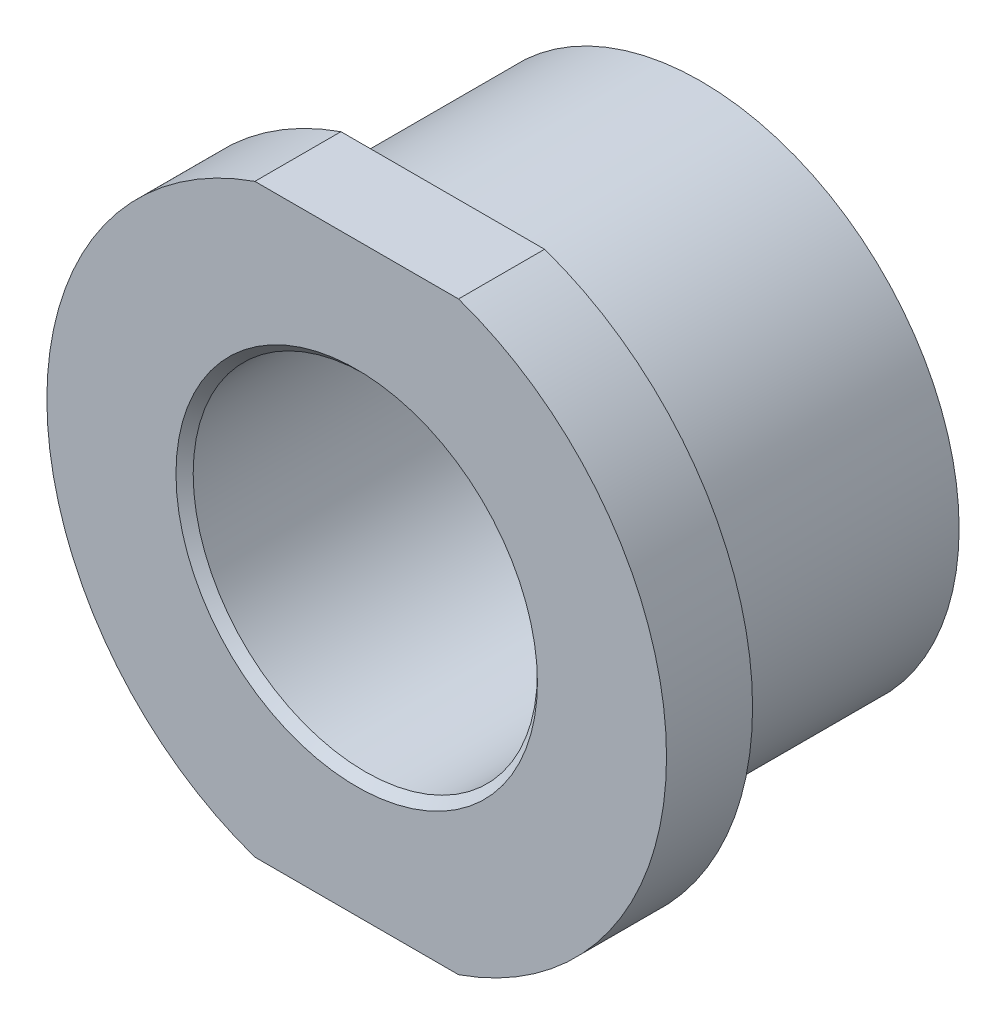
SolidWorks part; units mm, degrees
ref_plane "Front Plane" through (0, 0, 0) normal (0, 0, 1) x (1, 0, 0)
ref_plane "Top Plane" through (0, 0, 0) normal (0, 1, 0) x (1, 0, 0)
ref_plane "Right Plane" through (0, 0, 0) normal (1, 0, 0) x (0, 0, -1)
sketch "Sketch1" plane through (0, 0, 0) normal (0, 0, 1) x (1, 0, 0)
  circle A0 centre (0, 0) radius 15
  circle A1 centre (0, 0) radius 10
  dimension "D1" = 30
  dimension "D2" = 20
extrude "Boss-Extrude1" add sketch "Sketch1" along normal blind 15
sketch "Sketch2" plane through (0, 0, 15) normal (0, 0, 1) x (1, 0, 0)
  line L0 (-5.9161, 17) -> (5.9161, 17)
  line L1 (-5.9161, -17) -> (5.9161, -17)
  circle A0 centre (0, 0) radius 10 construction
  circle A1 centre (0, 0) radius 10
  arc A2 (-5.9161, 17) -> (-5.9161, -17) centre (0, 0) ccw
  arc A3 (5.9161, -17) -> (5.9161, 17) centre (0, 0) ccw
  dimension "D1" = 36
  dimension "D2" = 34
  dimension "D3" = 17
extrude "Boss-Extrude2" add sketch "Sketch2" along normal blind 5
chamfer "Chamfer1" distance 0.5 angle 45 2 edges at (10, 0, 0) (10, 0, 20)
